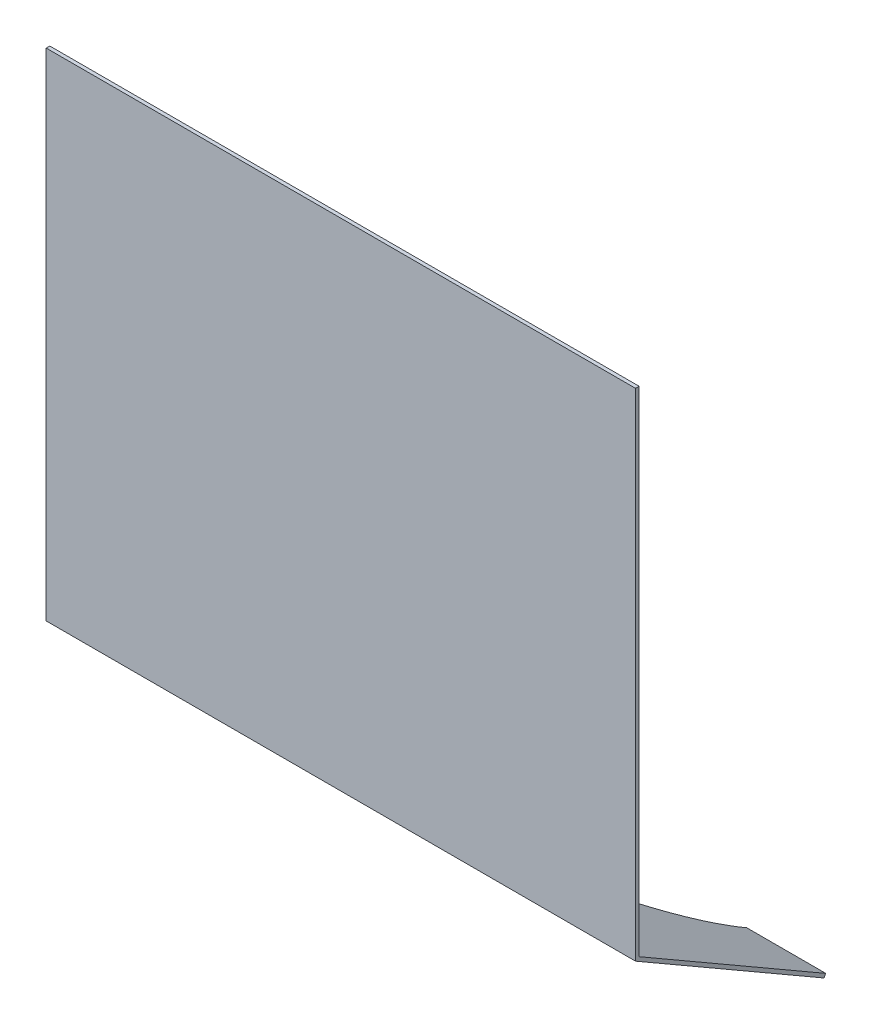
from build123d import *

# Parameters (mm, degrees)
SKETCH_1_W          = 328
SKETCH_1_H          = 275
EXTRUDE_1_DEPTH     = 2
EXTRUDE_2_DEPTH     = 328
SKETCH_4_RX         = 120
SKETCH_4_RY         = 100
CUT_EXTRUDE_1_DEPTH = 10


with BuildPart() as part:
    # 草图1 → 凸台-拉伸1 (new body)
    with BuildSketch(Plane.XY):
        Rectangle(SKETCH_1_W, SKETCH_1_H)
    extrude(amount=EXTRUDE_1_DEPTH)

    # 草图2 → 凸台-拉伸2 (add)
    with BuildSketch(Plane.ZY.offset(164)):
        Polygon((0, -137.5), (-103.923048454, -197.5), (-102.923048454, -199.232050808), (1, -139.232050808), (2, -138.654700538), (2, -137.5), align=None)
    extrude(amount=-EXTRUDE_2_DEPTH)

    # 草图4 → 切除-拉伸1 (cut)
    with BuildSketch(Plane(origin=(0, -103.125, 59.53924651), x_dir=(1, 0, 0), z_dir=(0, 0.8660254037844398, -0.49999999999999784))):
        with Locations(Location((0, 188.75), (0, 0, 0))):
            Ellipse(SKETCH_4_RX, SKETCH_4_RY)
    extrude(amount=-CUT_EXTRUDE_1_DEPTH, mode=Mode.SUBTRACT)


solid = part.part
